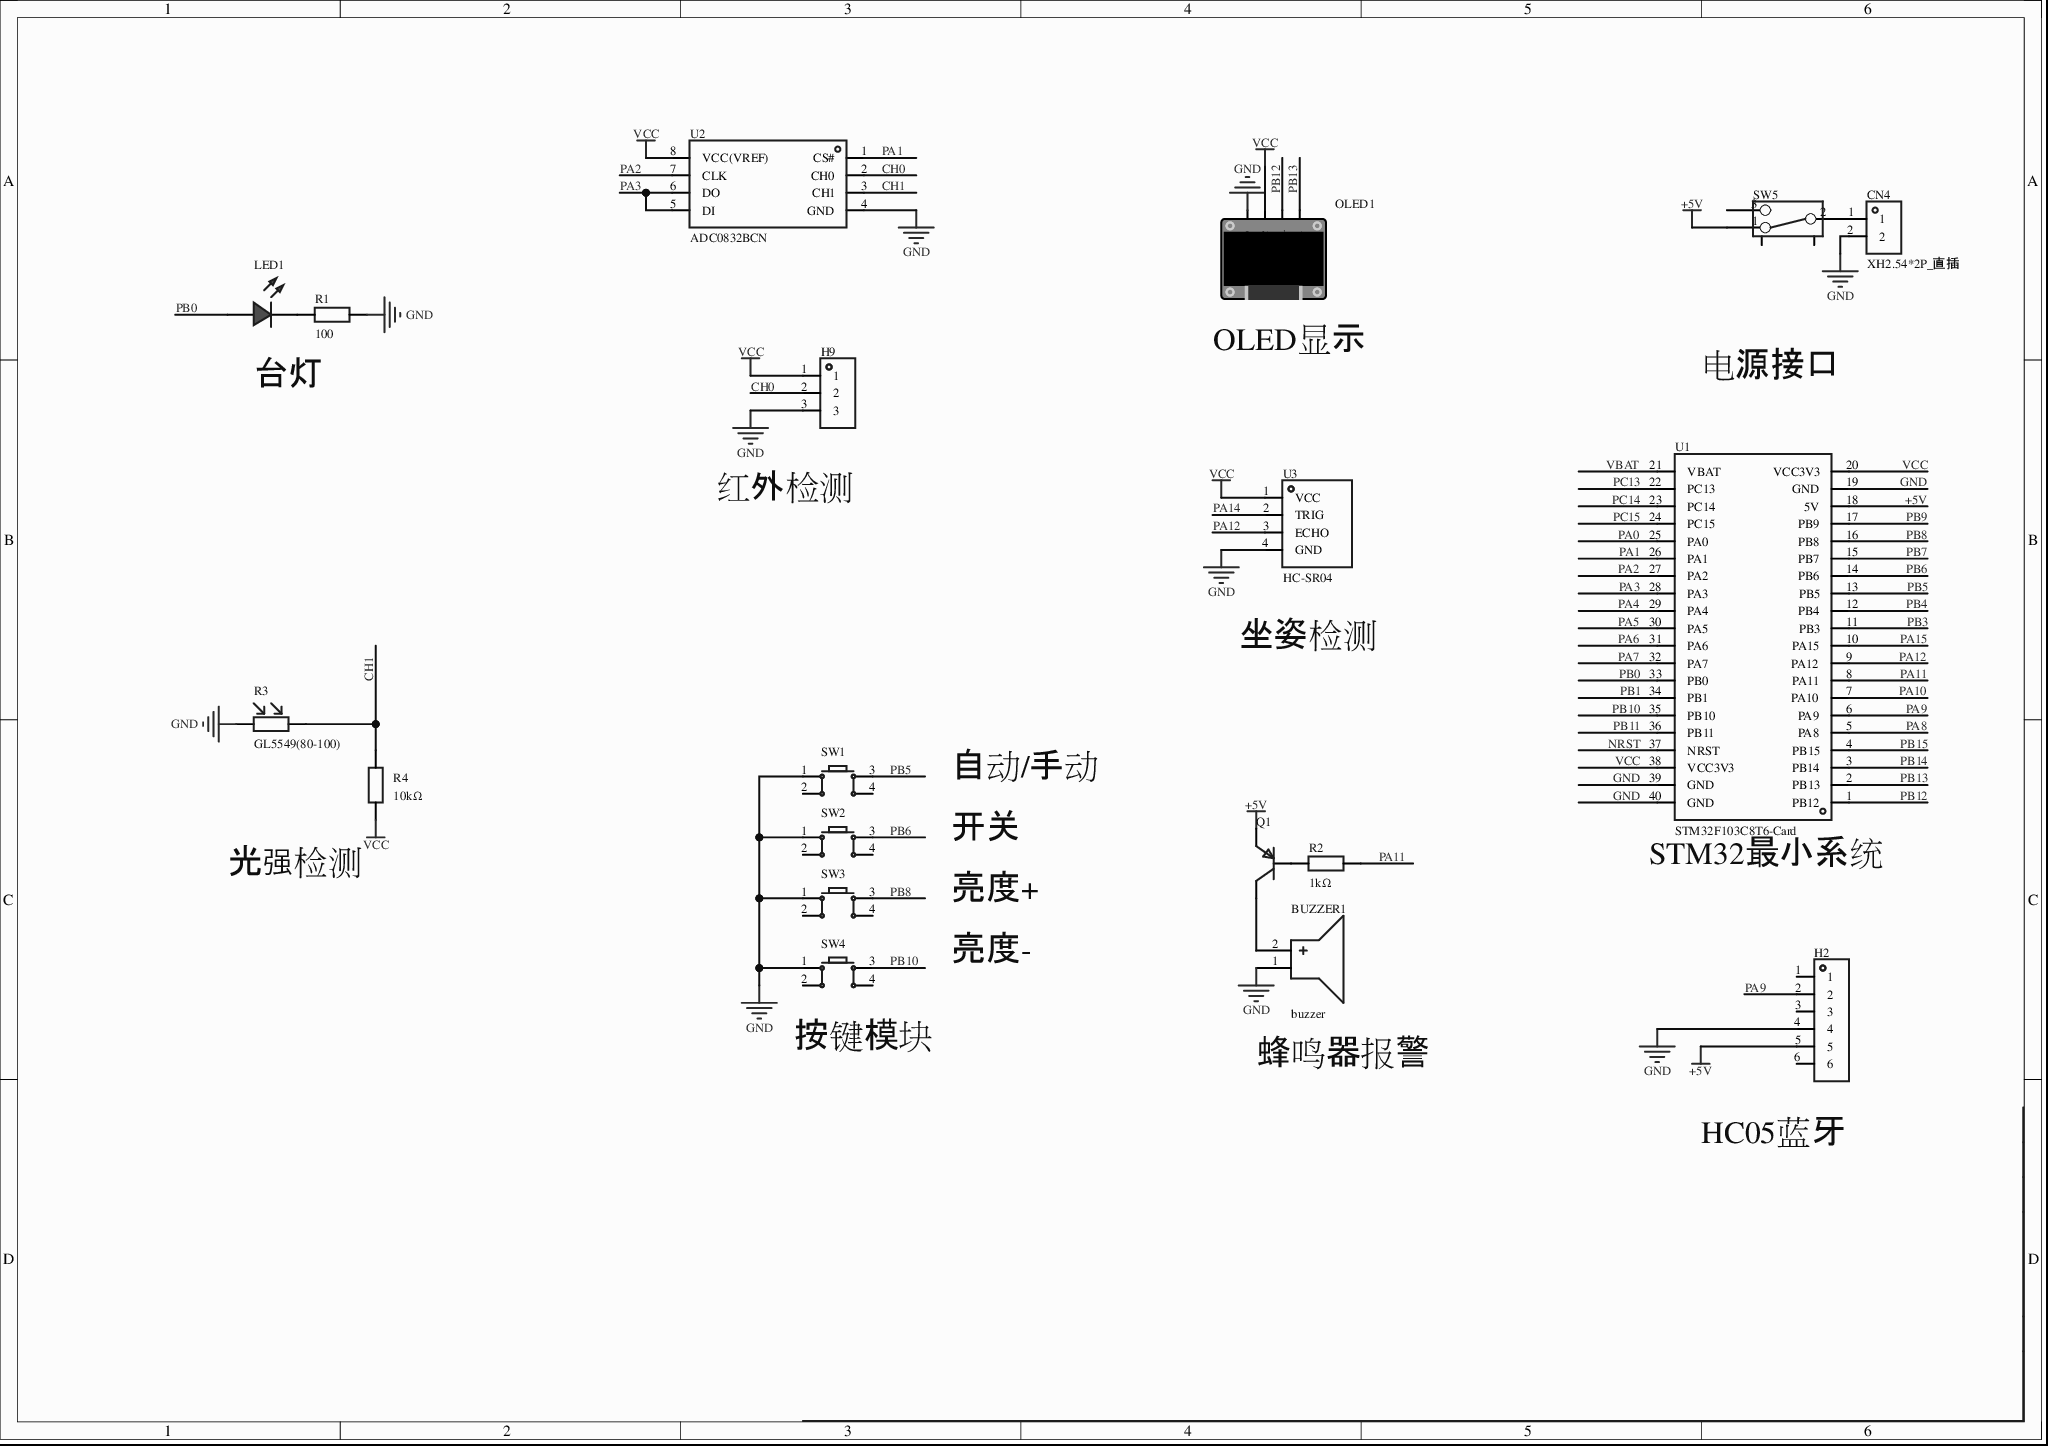
[diagram p0: MISC51796-3.schdoc]
# Altium project MISC51796-2.PrjPcb
1 sheet, 19 parts. Net scope: global (net labels, ports and power ports of the same name join across sheets).
Board file: MISC51796.pcbdoc

## Sheet MISC51796-3.schdoc
size 297 x 209 mm; Version: V1.0; @Project Name: MISC51796; @Page Count: 1; @Update Date: 2026-04-24; @Create Date: 2026-04-24; @Schematic Name: MISC51796; @Page No: 1; @Create Time: 23:22:16; @Update Time: 17:32:40; @Board Name: MISC51796

### Parts
BUZZER1  buzzer  [BUZ-TH_BD12.0-P6.00-D0.9-RD]
CN4  XH2.54*2P_直插  [CONN-TH_2P-P2.50-XH2.54-2P]
H2  (no value)  [HDR-TH_6P-P2.54-V-F]
H9  (no value)  [HDR-TH_3P-P2.54-V-F]
LED1  (no value)  [LED_TH-3mm]
OLED1  (no value)  [0.96OLED_4P]
Q1  (no value)  [S8550P_TO-92]
R1  100  [Res_1/8W]
R2  1kΩ  [Res_1/8W]
R3  GL5549(80-100)  [RES-TH_L5.1-W4.3-P3.40-D0.5]
R4  10kΩ  [Res_1/8W]
SW1  (no value)  [SW-TH_4P-L6.0-W6.0-P4.50-LS6.5]
SW2  (no value)  [SW-TH_4P-L6.0-W6.0-P4.50-LS6.5]
SW3  (no value)  [SW-TH_4P-L6.0-W6.0-P4.50-LS6.5]
SW4  (no value)  [SW-TH_4P-L6.0-W6.0-P4.50-LS6.5]
SW5  (no value)  [拨动开关]
U1  STM32F103C8T6-Card  [CONN-TH_L53.3-W22.9_STM32F103C8T6-CARD]
U2  ADC0832BCN  [PDIP-8_L9.6-W6.4-P2.54-LS7.6-BL]
U3  HC-SR04  [TH_HC-SR04V]

### Nets
+5V: H2.5 Q1.1(E) SW5.1 U1.18(5V)
GND: BUZZER1.1(-) CN4.2 H2.4 H9.3 OLED1.1(GND) R1.2 R3.1 SW1.1 SW2.1 SW3.1 SW4.1 U1.19(GND) U1.39(GND) U1.40(GND) U2.4(GND) U3.4(GND)
VCC: H9.1 OLED1.2(VCC) R4.1 U1.20(VCC3V3) U1.38(VCC3V3) U2.8(VCC(VREF)) U3.1(VCC)
CH0: H9.2 U2.2(CH0)
CH1: R3.2 R4.2 U2.3(CH1)
NRST: U1.37(NRST)
PA0: U1.25(PA0)
PA1: U1.26(PA1) U2.1(CS#)
PA2: U1.27(PA2) U2.7(CLK)
PA3: U1.28(PA3) U2.5(DI) U2.6(DO)
PA4: U1.29(PA4)
PA5: U1.30(PA5)
PA6: U1.31(PA6)
PA7: U1.32(PA7)
PA8: U1.5(PA8)
PA9: H2.2 U1.6(PA9)
PA10: U1.7(PA10)
PA11: R2.2 U1.8(PA11)
PA12: U1.9(PA12) U3.3(ECHO)
PA14: U3.2(TRIG)
PA15: U1.10(PA15)
PB0: LED1.1(C) U1.33(PB0)
PB1: U1.34(PB1)
PB3: U1.11(PB3)
PB4: U1.12(PB4)
PB5: SW1.3 U1.13(PB5)
PB6: SW2.3 U1.14(PB6)
PB7: U1.15(PB7)
PB8: SW3.3 U1.16(PB8)
PB9: U1.17(PB9)
PB10: SW4.3 U1.35(PB10)
PB11: U1.36(PB11)
PB12: OLED1.3(SCL) U1.1(PB12)
PB13: OLED1.4(SDA) U1.2(PB13)
PB14: U1.3(PB14)
PB15: U1.4(PB15)
PC13: U1.22(PC13)
PC14: U1.23(PC14)
PC15: U1.24(PC15)
VBAT: U1.21(VBAT)
NetBUZZER1_2: BUZZER1.2(+) Q1.3(C)
NetCN4_1: CN4.1 SW5.2
NetLED1_2: LED1.2(A) R1.1
NetQ1_2: Q1.2(B) R2.1

Not connected (* = marked no-connect by the designer): H2 1 3 6; SW1 2 4; SW2 2 4; SW3 2 4; SW4 2 4; SW5 3 4 5

### Notes on the sheet
- 台灯
- OLED显示
- 电源接口
- 红外检测
- 坐姿检测
- 自动/手动
- 开关
- (near U1) STM32最小系统
- 光强检测
- 亮度+
- 亮度-
- (near SW4) 按键模块
- 蜂鸣器报警
- (near H2) HC05蓝牙

### Library data of the parts
BUZZER1 = buzzer: AddInBom: yes; ModelId: af17e4151ed84fc2a628230bf23763630819f05c4eef4c71ace90d822a990e87; ModelTransform: 472.44,472.176,0,270,0,0,0,0,-196.85; Symbol: BUZZER; Device: buzzer; LCSC Part Name: buzzer; SupplierPart: C9900014030; ManufacturerPart: buzzer; Supplier Footprint: buzzer; JLCPCB Part Class: Extended Part; Supplier: LCSC; ConvertToPcb: yes; FootprintName: BUZ-TH_BD12.0-P6.00-D0.9-RD; ModelName: BUZ-TH_BD12.0-P6.00-D0.9-RD
CN4 = XH2.54*2P_直插: 3D Model: 325c595e30db4df8abe76612dd40b0fa0819f05c4eef4c71ace90d822a990e87; 3D Model Transform: 295.275,228.346,0,180,0,0,-0.002,-20.079,-137.795; AddInBom: yes; Device: XH2.54*2P_直插; Symbol: XH2.54*2P_直插; LCSC Part Name: XH2.54*2P_直插; Supplier Part: C9900008615; Manufacturer Part: XH2.54*2P_直插; Supplier Footprint: XH2.54_2P; JLCPCB Part Class: Extended Part; Supplier: LCSC; FootprintName: CONN-TH_2P-P2.50-XH2.54-2P; ConvertToPcb: yes; ModelName: CONN-TH_2P-P2.50-XH2.54-2P
H2 = HDR-F_2.54_1x6P: Symbol: Header-Female-2.54_1x6; ConvertToPcb: yes; ModelId: 0f5bcf94dcda47d085f24cdca1696fe9; ModelTransform: 619.684,94.488,0,0,0,0,0,0,-125.984; Device: HDR-F_2.54_1x6P; AddInBom: yes; SupplierPart: C40877; Supplier Footprint: 插件; FootprintName: HDR-TH_6P-P2.54-V-F; ModelName: HDR-TH_6P-P2.54-V-F
H9 = HDR-F_2.54_1x3P: Symbol: PM254V-11-03-H85; ConvertToPcb: yes; ModelId: f3b3cc5aae9641bf9e56fc160cef875b; ModelName: HDR2.54-F-LI-1X3P; ModelTransform: 299.9994,100,0,0,0,0,0,0,-118.11; Device: HDR-F_2.54_1x3P; AddInBom: yes; SupplierPart: C541850; Supplier Footprint: 插件; FootprintName: HDR-TH_3P-P2.54-V-F
LED1 = LED_TH-R_3mm: ConvertToPcb: yes; ModelId: a497c992633541038a38947cdc58012f0819f05c4eef4c71ace90d822a990e87; ModelName: LED-TH-3mm_R; ModelTransform: 141.274,153.327,0,0,0,0,-5.984,0,-137.795; Symbol: LED_TH-R; Device: LED_TH-R_3mm; AddInBom: yes; FootprintName: LED_TH-3mm; Supplier Footprint: 插件
OLED1 = 0.96OLED模块_4P: 3D Model: 79c000fdb68d45a296c2e9bedf4f9055; 3D Model Transform: 1393.69792,1318.895,0,0,0,0,0,-560.079,-137.795; ConvertToPcb: yes; Symbol: 0.96OLED模块_4P; Device: 0.96OLED模块_4P; Supplier Footprint: 插件; AddInBom: yes; FootprintName: 0.96OLED_4P; ModelName: 0.96OLED_4P
Q1 = S8550_TO_PNP: ConvertToPcb: yes; ModelId: aafe8e06f2154e7c93506efd0d6632dd0819f05c4eef4c71ace90d822a990e87; ModelName: TO-92-3_L4.9-W3.7-P1.27-L; ModelTransform: 180.78,141.44,417.3,0,0,0,0,0,-200; Symbol: S8550_TO_PNP; Device: S8550_TO_PNP; AddInBom: yes; Supplier Footprint: TO-92; FootprintName: S8550P_TO-92
R1 = Res_AXIAL-1/8W: Symbol: 电阻; ConvertToPcb: yes; ModelId: b2b5ae7ae4c642178fe0039925c86a3f0819f05c4eef4c71ace90d822a990e87; ModelName: RES-TH_BD1.8-L3.2-P7.20-D0.4; ModelTransform: 282.86,66.88,253.09,0,0,0,0,0,-191; Device: Res_AXIAL-1/8W; Value: 100; AddInBom: yes; Supplier Footprint: 轴向引线; FootprintName: Res_1/8W
R2 R4 = Res_AXIAL-1/8W: Symbol: 电阻; 3D Model: b2b5ae7ae4c642178fe0039925c86a3f0819f05c4eef4c71ace90d822a990e87; 3D Model Transform: 282.86,66.88,253.09,0,0,0,0,0,-191; ConvertToPcb: yes; ModelName: RES-TH_BD1.8-L3.2-P7.20-D0.4; Device: Res_AXIAL-1/8W; Supplier Footprint: 轴向引线; AddInBom: yes; FootprintName: Res_1/8W
  R2: Value: 1kΩ
  R4: Value: 10kΩ
R3 = GL5549(80-100): 暗电阻:20MΩ;亮电阻@10Lux:80kΩ~150kΩ;光谱峰值(波长):540nm;; Manufacturer: JCHL(晶创和立); AddInBom: yes; ModelId: cb75fcf2d6c94cac811f2579121b87200819f05c4eef4c71ace90d822a990e87; ModelTransform: 169.291,200.39669,0,0,0,0,-3.937,0,-137.795; Dark Resistance: 20MΩ; Voltage - Max: 150V; Wavelength - Peak: 540nm; γ Value: 0.8; Pitch: 3.4mm; Symbol: GL5549(80-100); Device: GL5549(80-100); LCSC Part Name: 光敏电阻性能参数; SupplierPart: C10078; ManufacturerPart: GL5549(80-100); Supplier Footprint: 插件,P=3.4mm; JLCPCB Part Class: Extended Part; Datasheet: https://item.szlcsc.com/datasheet/GL5549(80-100)/10617.html; Supplier: LCSC; ConvertToPcb: yes; FootprintName: RES-TH_L5.1-W4.3-P3.40-D0.5; ModelName: RES-TH_L5.1-W4.3-P3.40-D0.5; Cell Resistance @ Illuminance: 80kΩ~150kΩ; Operating Temperature: -30℃~+70℃; Length: 5.1mm; Width: 4.3mm; Height: 2.4mm
SW1-SW4 = Key_TH_6x6x6: 触点电流:50mA;额定电压(DC):12V;绝缘电阻:100MΩ;电路结构:单刀单掷;安装方式:直插;按钮形状:圆形按钮;按钮/盖帽颜色:黑色;作用力:260gf@±30gf;工作温度:-25℃~+70℃;引脚样式:PC引脚;开关长度:6mm;开关宽度:6mm;开关高度:6mm;带支架:否;; Symbol: 轻触按键; AddInBom: yes; ModelId: 20eee248bc684ccd8cbdbb1d0d91ec6f0819f05c4eef4c71ace90d822a990e87; ModelName: SW-TH_4P-L6.0-W6.0-H5.0-LS6.5-P4.50; ModelTransform: 236.22,323.03,0,90,0,0,0,0,-137.795; Device: Key_TH_6x6x6; FootprintName: SW-TH_4P-L6.0-W6.0-P4.50-LS6.5; ConvertToPcb: yes; Supplier Footprint: 插件
SW5 = 拨动开关_正: ConvertToPcb: yes; ModelId: 4321fe59a4074cbfb4989553f297c68f0819f05c4eef4c71ace90d822a990e87; ModelName: SW-TH_SS-12D02-VG4; ModelTransform: 370.09,208.7,472.35,0,0,0,0,0,-110; Device: 拨动开关_正; Symbol: 拨动开关; FootprintName: 拨动开关; AddInBom: yes; Supplier Footprint: 插件
U1 = STM32F103C8T6-Card: AddInBom: yes; Device: STM32F103C8T6-Card; Symbol: STM32F103C8T6-CARD; FootprintName: CONN-TH_L53.3-W22.9_STM32F103C8T6-CARD; LCSC Part Name: STM32F103C8T6-Card; SupplierPart: C9900077949; ManufacturerPart: STM32F103C8T6-Card; Supplier Footprint: 插件; Supplier: LCSC; ConvertToPcb: yes
U2 = ADC0832BCN: 分辨率:8位;工作电压:4.5V~6.3V;; Manufacturer: TI(德州仪器); AddInBom: yes; ModelId: 5dc2af053da0476fab11ee64b9a10a940819f05c4eef4c71ace90d822a990e87; ModelName: PDIP-8_L9.6-W6.4-P2.54-LS7.62-BL; ModelTransform: 377.952,309.842,0,0,0,0,0,0,-137.795; Resolution(Bits): 8位; number of channels: 2; Symbol: ADC0832BCN; Device: ADC0832BCN; LCSC Part Name: ADC0832BCN; SupplierPart: C17246630; ManufacturerPart: ADC0832BCN; Supplier Footprint: MDIP-8; JLCPCB Part Class: Extended Part; Datasheet: https://item.szlcsc.com/datasheet/ADC0832BCN/18375746.html; Supplier: LCSC; ConvertToPcb: yes; FootprintName: PDIP-8_L9.6-W6.4-P2.54-LS7.6-BL; Voltage - Supply: 4.5V~6.3V; differential input: -; Operating Temperature: -40℃~+85℃
U3 = HC-SR04: Manufacturer: Universal Microelectronics; AddInBom: yes; Symbol: HC-SR04; Device: HC-SR04; LCSC Part Name: HC-SR04; SupplierPart: C19857336; ManufacturerPart: HC-SR04; Supplier Footprint: -; JLCPCB Part Class: 扩展库; Datasheet: https://atta.szlcsc.com/upload/public/pdf/source/20240122/47B8E374E428935B7962A2189EF91AAC.pdf; Supplier: LCSC; ConvertToPcb: yes; FootprintName: TH_HC-SR04V